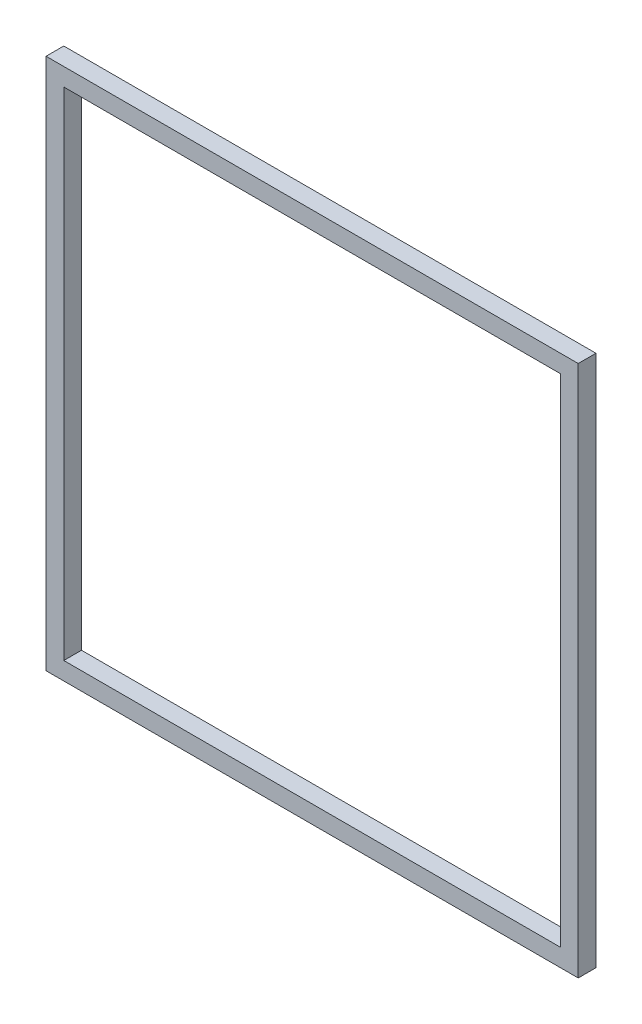
SolidWorks part; units mm, degrees
ref_plane "前视基准面" through (0, 0, 0) normal (0, 0, 1) x (1, 0, 0)
ref_plane "上视基准面" through (0, 0, 0) normal (0, 1, 0) x (1, 0, 0)
ref_plane "右视基准面" through (0, 0, 0) normal (1, 0, 0) x (0, 0, -1)
other "Configuration Table"
sketch "草图1" plane through (0, 0, 0) normal (0, 0, 1) x (1, 0, 0)
  line L0 (-150, -150) -> (150, -150)
  line L1 (150, -150) -> (150, 150)
  line L2 (150, 150) -> (-150, 150)
  line L3 (-150, 150) -> (-150, -150)
  line L4 (-140, -140) -> (140, -140)
  line L5 (140, -140) -> (140, 140)
  line L6 (140, 140) -> (-140, 140)
  line L7 (-140, 140) -> (-140, -140)
  point P0 (0, 0)
  dimension "D1" = 10
  dimension "D2" = 150
  dimension "D3" = 290
  dimension "D4" = 300
  dimension "D5" = 10
  dimension "D6" = 150
  dimension "D7" = 290
  dimension "D8" = 300
extrude "凸台-拉伸1" add sketch "草图1" against normal mid plane 10
